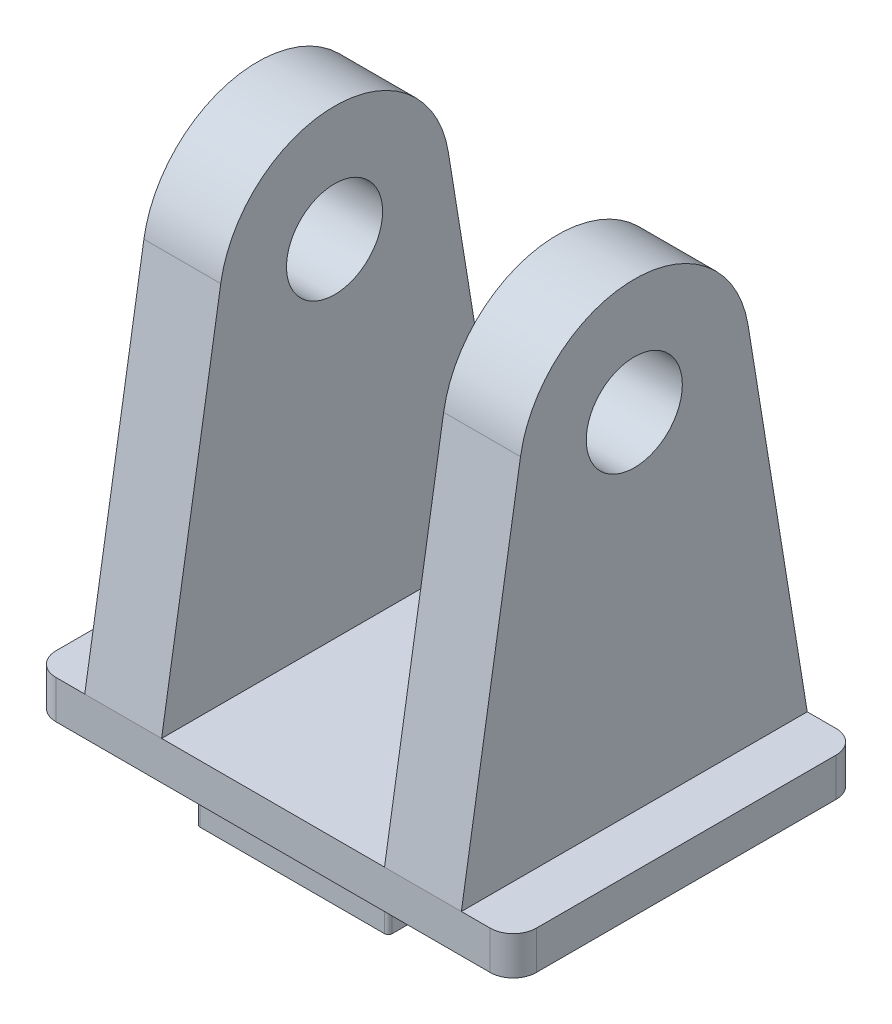
SolidWorks part; units mm, degrees
ref_plane "Front Plane" through (0, 0, 0) normal (0, 0, 1) x (1, 0, 0)
ref_plane "Top Plane" through (0, 0, 0) normal (0, 1, 0) x (1, 0, 0)
ref_plane "Right Plane" through (0, 0, 0) normal (1, 0, 0) x (0, 0, -1)
sketch "Sketch 1" plane through (0, 0, 0) normal (0, 1, 0) x (1, 0, 0)
  line L0 (0, 180.7895) -> (0, -186.3158) construction
  line L1 (-167.3684, 0) -> (124.7368, 0) construction
  line L2 (113, 90) -> (-113, 90)
  line L3 (-125, 78) -> (-125, -78)
  line L4 (125, 78) -> (125, -78)
  line L5 (113, -90) -> (-113, -90)
  arc A0 (-113, 90) -> (-125, 78) centre (-113, 78) ccw
  arc A1 (113, 90) -> (125, 78) centre (113, 78) cw
  arc A2 (113, -90) -> (125, -78) centre (113, -78) ccw
  arc A3 (-113, -90) -> (-125, -78) centre (-113, -78) cw
  point P8 (0, -90)
  point P13 (-125, 0)
  point P14 (0, 90)
  point P20 (125, 0)
  dimension "D3" = 12
  dimension "D1" = 250
  dimension "D2" = 180
extrude "Boss-Extrude 1" add sketch "Sketch 1" along normal blind 20
sketch "Sketch 2" plane through (0, 0, 0) normal (0, -1, 0) x (1, 0, 0)
  line L0 (0, 115.2814) -> (0, -122.6629) construction
  line L1 (-106.8144, 0) -> (93.7883, 0) construction
  line L2 (48, 80) -> (-48, 80)
  line L3 (-50, 78) -> (-50, -78)
  line L4 (-113, 90) -> (113, 90) construction
  line L5 (50, 78) -> (50, -78)
  line L6 (48, -80) -> (-48, -80)
  arc A0 (-48, 80) -> (-50, 78) centre (-48, 78) ccw
  arc A1 (48, 80) -> (50, 78) centre (48, 78) cw
  arc A2 (48, -80) -> (50, -78) centre (48, -78) ccw
  arc A3 (-48, -80) -> (-50, -78) centre (-48, -78) cw
  point P8 (0, -80)
  point P15 (-50, 0)
  point P16 (0, 80)
  point P22 (50, 0)
  dimension "D1" = 2
  dimension "D2" = 10
  dimension "D3" = 100
extrude "Boss-Extrude 2" add sketch "Sketch 2" along normal blind 20
sketch "Sketch 3" plane through (0, 0, 0) normal (1, 0, 0) x (0, 0, -1)
  line L0 (0, 284.2134) -> (0, -75.8484) construction
  line L1 (-59.225, 209.6125) -> (-90, 20)
  line L2 (-90, 20) -> (90, 20)
  line L3 (-78, 20) -> (78, 20) construction
  line L4 (59.225, 209.6125) -> (90, 20)
  line L5 (78, 0) -> (-78, 0) construction
  arc A0 (59.225, 209.6125) -> (-59.225, 209.6125) centre (0, 200) ccw
  circle A1 centre (0, 200) radius 25
  point P12 (0, 20)
  dimension "D1" = 50
  dimension "D2" = 60
  dimension "D3" = 200
extrude "Boss-Extrude 3" add sketch "Sketch 3" along normal blind 40 from offset 58
mirror "Mirror 1" about plane through (0, 0, 0) normal (1, 0, 0) of "Boss-Extrude 3"
